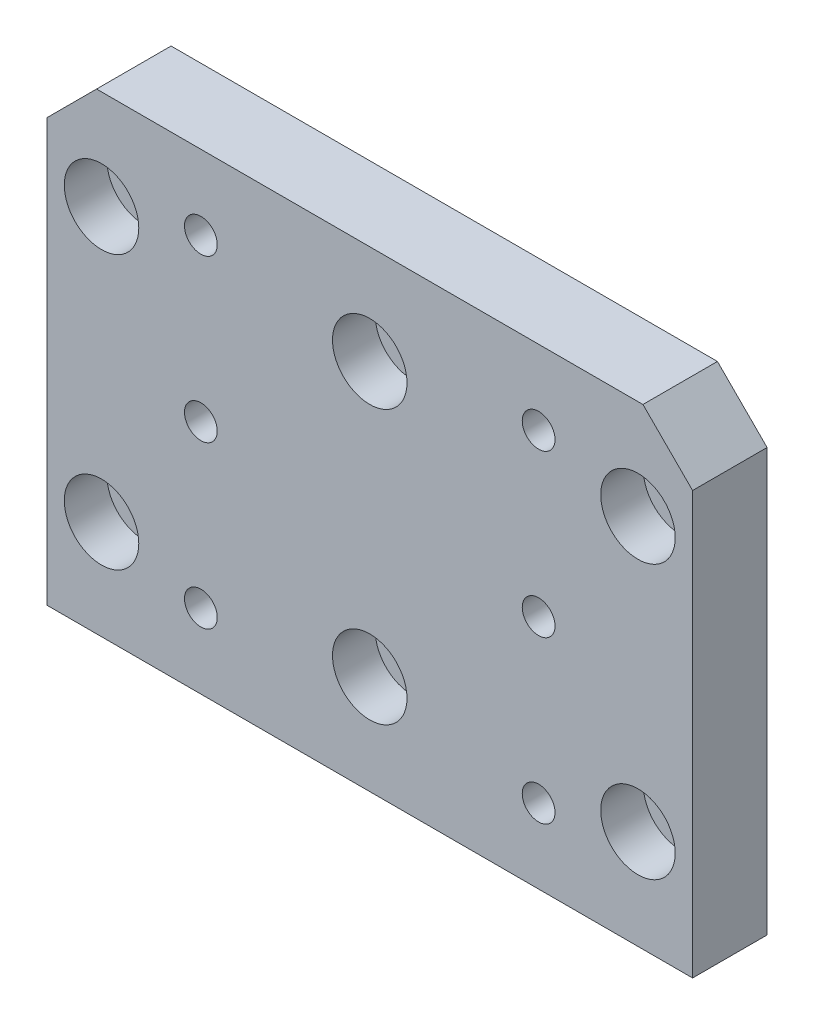
SolidWorks part; units mm, degrees
ref_plane "Front Plane" through (0, 0, 0) normal (0, 0, 1) x (1, 0, 0)
ref_plane "Top Plane" through (0, 0, 0) normal (0, 1, 0) x (1, 0, 0)
ref_plane "Right Plane" through (0, 0, 0) normal (1, 0, 0) x (0, 0, -1)
sketch "Sketch1" plane through (0, 0, 0) normal (0, 0, 1) x (1, 0, 0)
  line L1 (-65, 47.5) -> (65, 47.5)
  line L2 (-65, 47.5) -> (-65, -47.5)
  line L3 (-65, -47.5) -> (65, -47.5)
  line L4 (65, 47.5) -> (65, -47.5)
  line L5 (-65, 47.5) -> (65, -47.5) construction
  line L6 (-65, -47.5) -> (65, 47.5) construction
  point P0 (0, 0)
  dimension "D1" = 95
  dimension "D2" = 130
extrude "Boss-Extrude1" add sketch "Sketch1" along normal blind 15
hole_wizard "CBORE for M8 Hex Socket Head Cap Screw1" positions "Sketch5" profile "Sketch4" counterbore size "M8" standard "Iso" end condition through all
sketch "Sketch5" plane through (0, 0, 15) normal (0, 0, 1) x (1, 0, 0)
  line L0 (0, 0) -> (106.8837, 0) construction
  line L3 (0, 0) -> (0, -87.1362) construction
  point P0 (54, 27.5)
  point P2 (54, -27.5)
  point P4 (-54, 27.5)
  point P6 (-54, -27.5)
  point P19 (0, 27.5)
  point P21 (0, -27.5)
  dimension "D1" = 55
  dimension "D2" = 108
sketch "Sketch4" plane through (54, 27.5, 15) normal (1, 0, 0) x (0, -1, 0)
  line L0 (0, 0) -> (0, 15)
  line L1 (0, 15) -> (4.5, 15)
  line L3 (4.5, 15) -> (4.5, 8.6)
  line L4 (4.5, 8.6) -> (7.5, 8.6)
  line L5 (7.5, 8.6) -> (7.5, 0)
  line L7 (7.5, 0) -> (0, 0)
  line L11 (0, -6.35) -> (0, 107.95) construction
  dimension "通孔孔直径" = 9
  dimension "通孔孔深度" = 15
  dimension "柱形沉头孔直径" = 15
  dimension "柱形沉头孔深度" = 8.6
chamfer "Chamfer1" distance 10 angle 45 2 edges at (65, 47.5, 7.5) (-65, 47.5, 7.5)
hole_wizard "CBORE for M6 Hex Socket Head Cap Screw1" positions "Sketch7" profile "Sketch6" counterbore size "M6" standard "Iso" end condition through all
sketch "Sketch7" plane through (0, 0, 0) normal (0, 0, -1) x (-1, 0, 0)
  line L0 (31.5, -32.5) -> (36.5, -32.5) construction
  point P0 (-34, -32.5)
  point P3 (-34, 0)
  point P6 (-34, 32.5)
  point P9 (34, -32.5)
  point P13 (34, 0)
  point P16 (34, 32.5)
sketch "Sketch6" plane through (34, -32.5, 0) normal (1, 0, 0) x (0, 1, 0)
  line L0 (0, 0) -> (0, 15)
  line L1 (0, 15) -> (3.3, 15)
  line L3 (3.3, 15) -> (3.3, 6.4)
  line L4 (3.3, 6.4) -> (5.5, 6.4)
  line L5 (5.5, 6.4) -> (5.5, 0)
  line L7 (5.5, 0) -> (0, 0)
  line L11 (0, -6.35) -> (0, 107.95) construction
  dimension "通孔孔直径" = 6.6
  dimension "通孔孔深度" = 15
  dimension "柱形沉头孔直径" = 11
  dimension "柱形沉头孔深度" = 6.4
